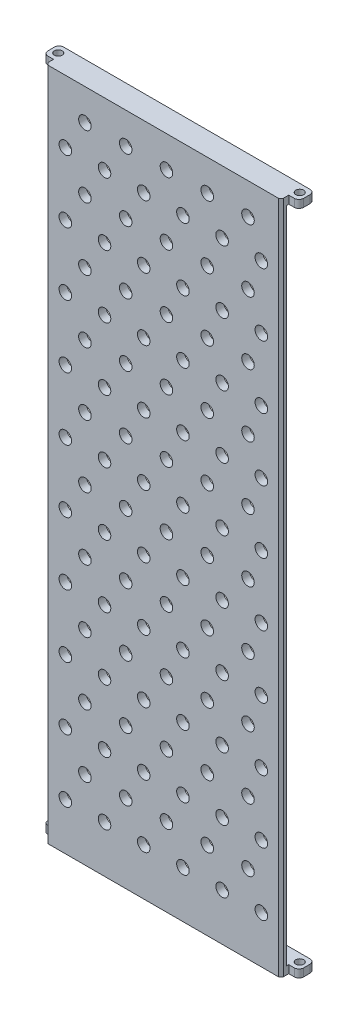
from build123d import *

# Parameters (mm, degrees)
SKETCH1_W               = 150
SKETCH1_H               = 420
BOSS_EXTRUDE1_DEPTH     = 5
CUT_EXTRUDE1_REACH      = 448.01
SKETCH2_R               = 4
LPATTERN1_COUNT         = 10
LPATTERN1_PITCH         = 40
BOSS_EXTRUDE2_DEPTH     = 5
BOSS_EXTRUDE3_DEPTH     = 5
CUT_EXTRUDE2_DEPTH      = 458.703233548
CUT_EXTRUDE2_DEPTH_BACK = 458.703233548
SKETCH6_R               = 2.5
SKETCH6_W               = 6.5
SKETCH6_H               = 5
FILLET1_R               = 3
CHAMFER1_SIZE           = 1.5


with BuildPart() as part:
    # Sketch1 → Boss-Extrude1 (new body)
    with BuildSketch(Plane.XY):
        with Locations((75, 210)):
            Rectangle(SKETCH1_W, SKETCH1_H)
    extrude(amount=BOSS_EXTRUDE1_DEPTH)

    # Sketch2 → Cut-Extrude1 (cut, up to next)
    with BuildSketch(Plane.XY.offset(5), mode=Mode.PRIVATE) as cut_extrude1_sk1:
        with Locations((25, 405)):
            Circle(SKETCH2_R)
    cut_extrude1_tool1 = extrude(cut_extrude1_sk1.sketch, amount=-CUT_EXTRUDE1_REACH, mode=Mode.PRIVATE) & part.part
    # Sketch2 → Cut-Extrude1 (cut, up to next)
    with BuildSketch(Plane.XY.offset(5), mode=Mode.PRIVATE) as cut_extrude1_sk2:
        with Locations((51, 405)):
            Circle(SKETCH2_R)
    cut_extrude1_tool2 = extrude(cut_extrude1_sk2.sketch, amount=-CUT_EXTRUDE1_REACH, mode=Mode.PRIVATE) & part.part
    # Sketch2 → Cut-Extrude1 (cut, up to next)
    with BuildSketch(Plane.XY.offset(5), mode=Mode.PRIVATE) as cut_extrude1_sk3:
        with Locations((77, 405)):
            Circle(SKETCH2_R)
    cut_extrude1_tool3 = extrude(cut_extrude1_sk3.sketch, amount=-CUT_EXTRUDE1_REACH, mode=Mode.PRIVATE) & part.part
    # Sketch2 → Cut-Extrude1 (cut, up to next)
    with BuildSketch(Plane.XY.offset(5), mode=Mode.PRIVATE) as cut_extrude1_sk4:
        with Locations((103, 405)):
            Circle(SKETCH2_R)
    cut_extrude1_tool4 = extrude(cut_extrude1_sk4.sketch, amount=-CUT_EXTRUDE1_REACH, mode=Mode.PRIVATE) & part.part
    # Sketch2 → Cut-Extrude1 (cut, up to next)
    with BuildSketch(Plane.XY.offset(5), mode=Mode.PRIVATE) as cut_extrude1_sk5:
        with Locations((129, 405)):
            Circle(SKETCH2_R)
    cut_extrude1_tool5 = extrude(cut_extrude1_sk5.sketch, amount=-CUT_EXTRUDE1_REACH, mode=Mode.PRIVATE) & part.part
    # Sketch2 → Cut-Extrude1 (cut, up to next)
    with BuildSketch(Plane.XY.offset(5), mode=Mode.PRIVATE) as cut_extrude1_sk6:
        with Locations((12.5, 385)):
            Circle(SKETCH2_R)
    cut_extrude1_tool6 = extrude(cut_extrude1_sk6.sketch, amount=-CUT_EXTRUDE1_REACH, mode=Mode.PRIVATE) & part.part
    # Sketch2 → Cut-Extrude1 (cut, up to next)
    with BuildSketch(Plane.XY.offset(5), mode=Mode.PRIVATE) as cut_extrude1_sk7:
        with Locations((37.5, 385)):
            Circle(SKETCH2_R)
    cut_extrude1_tool7 = extrude(cut_extrude1_sk7.sketch, amount=-CUT_EXTRUDE1_REACH, mode=Mode.PRIVATE) & part.part
    # Sketch2 → Cut-Extrude1 (cut, up to next)
    with BuildSketch(Plane.XY.offset(5), mode=Mode.PRIVATE) as cut_extrude1_sk8:
        with Locations((62.5, 385)):
            Circle(SKETCH2_R)
    cut_extrude1_tool8 = extrude(cut_extrude1_sk8.sketch, amount=-CUT_EXTRUDE1_REACH, mode=Mode.PRIVATE) & part.part
    # Sketch2 → Cut-Extrude1 (cut, up to next)
    with BuildSketch(Plane.XY.offset(5), mode=Mode.PRIVATE) as cut_extrude1_sk9:
        with Locations((87.5, 385)):
            Circle(SKETCH2_R)
    cut_extrude1_tool9 = extrude(cut_extrude1_sk9.sketch, amount=-CUT_EXTRUDE1_REACH, mode=Mode.PRIVATE) & part.part
    # Sketch2 → Cut-Extrude1 (cut, up to next)
    with BuildSketch(Plane.XY.offset(5), mode=Mode.PRIVATE) as cut_extrude1_sk10:
        with Locations((112.5, 385)):
            Circle(SKETCH2_R)
    cut_extrude1_tool10 = extrude(cut_extrude1_sk10.sketch, amount=-CUT_EXTRUDE1_REACH, mode=Mode.PRIVATE) & part.part
    # Sketch2 → Cut-Extrude1 (cut, up to next)
    with BuildSketch(Plane.XY.offset(5), mode=Mode.PRIVATE) as cut_extrude1_sk11:
        with Locations((137.5, 385)):
            Circle(SKETCH2_R)
    cut_extrude1_tool11 = extrude(cut_extrude1_sk11.sketch, amount=-CUT_EXTRUDE1_REACH, mode=Mode.PRIVATE) & part.part
    cut_extrude1_1 = cut_extrude1_tool1.solids().sort_by_distance((25, 405, 5))[0]
    add(cut_extrude1_1, mode=Mode.SUBTRACT)
    cut_extrude1_2 = cut_extrude1_tool2.solids().sort_by_distance((51, 405, 5))[0]
    add(cut_extrude1_2, mode=Mode.SUBTRACT)
    cut_extrude1_3 = cut_extrude1_tool3.solids().sort_by_distance((77, 405, 5))[0]
    add(cut_extrude1_3, mode=Mode.SUBTRACT)
    cut_extrude1_4 = cut_extrude1_tool4.solids().sort_by_distance((103, 405, 5))[0]
    add(cut_extrude1_4, mode=Mode.SUBTRACT)
    cut_extrude1_5 = cut_extrude1_tool5.solids().sort_by_distance((129, 405, 5))[0]
    add(cut_extrude1_5, mode=Mode.SUBTRACT)
    cut_extrude1_6 = cut_extrude1_tool6.solids().sort_by_distance((12.5, 385, 5))[0]
    add(cut_extrude1_6, mode=Mode.SUBTRACT)
    cut_extrude1_7 = cut_extrude1_tool7.solids().sort_by_distance((37.5, 385, 5))[0]
    add(cut_extrude1_7, mode=Mode.SUBTRACT)
    cut_extrude1_8 = cut_extrude1_tool8.solids().sort_by_distance((62.5, 385, 5))[0]
    add(cut_extrude1_8, mode=Mode.SUBTRACT)
    cut_extrude1_9 = cut_extrude1_tool9.solids().sort_by_distance((87.5, 385, 5))[0]
    add(cut_extrude1_9, mode=Mode.SUBTRACT)
    cut_extrude1_10 = cut_extrude1_tool10.solids().sort_by_distance((112.5, 385, 5))[0]
    add(cut_extrude1_10, mode=Mode.SUBTRACT)
    cut_extrude1_11 = cut_extrude1_tool11.solids().sort_by_distance((137.5, 385, 5))[0]
    add(cut_extrude1_11, mode=Mode.SUBTRACT)
    cut_extrude1 = cut_extrude1_1 + cut_extrude1_2 + cut_extrude1_3 + cut_extrude1_4 + cut_extrude1_5 + cut_extrude1_6 + cut_extrude1_7 + cut_extrude1_8 + cut_extrude1_9 + cut_extrude1_10 + cut_extrude1_11  # Cut-Extrude1 as one shape, for the pattern or mirror that repeats it

    # LPattern1: Cut-Extrude1 ×10
    with Locations(*[(0, -i * LPATTERN1_PITCH, 0) for i in range(1, LPATTERN1_COUNT)]):
        add(cut_extrude1, mode=Mode.SUBTRACT)

    # Sketch3 → Boss-Extrude2 (add)
    with BuildSketch(Plane(origin=(0, 0, 0), x_dir=(-1, 0, 0), z_dir=(0, -1, 0))):
        Polygon((6.5, 10), (-156.5, 10), (-156.5, 0), (-150, 0), (-150, -5), (0, -5), (0, 0), (6.5, 0), align=None)
    extrude(amount=BOSS_EXTRUDE2_DEPTH)

    # Sketch4 → Boss-Extrude3 (add)
    with BuildSketch(Plane(origin=(0, 420, 0), x_dir=(1, 0, 0), z_dir=(0, 1, 0))):
        Polygon((150, -5), (150, 0), (156.5, 0), (156.5, 10), (-6.5, 10), (-6.5, 0), (0, 0), (0, -5), align=None)
    extrude(amount=BOSS_EXTRUDE3_DEPTH)

    # Sketch6 → Cut-Extrude2 (cut, two sides: drawn at the far end of the back side and taken through both)
    with BuildSketch(Plane(origin=(0, 425, 0), x_dir=(1, 0, 0), z_dir=(0, 1, 0)).offset(-CUT_EXTRUDE2_DEPTH_BACK)):
        with Locations(Location((-2, 5, 0), (0, 0, 90))):
            Circle(SKETCH6_R)
        with Locations(Location((152, 5, 0), (0, 0, 90))):
            Circle(SKETCH6_R)
        with Locations((153.25, -2.5)):
            Rectangle(SKETCH6_W, SKETCH6_H)
        with Locations((-3.25, -2.5)):
            Rectangle(SKETCH6_W, SKETCH6_H)
    extrude(amount=CUT_EXTRUDE2_DEPTH + CUT_EXTRUDE2_DEPTH_BACK, mode=Mode.SUBTRACT)

    # Fillet1
    fillet1_edges = [part.edges().sort_by_distance(p)[0] for p in [
        (-6.5, -2.5, 0),
        (-6.5, -2.5, -10),
        (156.5, -2.5, -10),
        (156.5, -2.5, 0),
        (-6.5, 422.5, -10),
        (-6.5, 422.5, 0),
        (156.5, 422.5, 0),
        (156.5, 422.5, -10),
    ]]
    fillet(fillet1_edges, radius=FILLET1_R)

    # Chamfer1
    chamfer1_edges = [part.edges().sort_by_distance(p)[0] for p in [
        (150, 210, 5),
        (0, 210, 5),
        (150, 210, 0),
        (0, 210, 0),
    ]]
    chamfer(chamfer1_edges, length=CHAMFER1_SIZE)


solid = part.part
